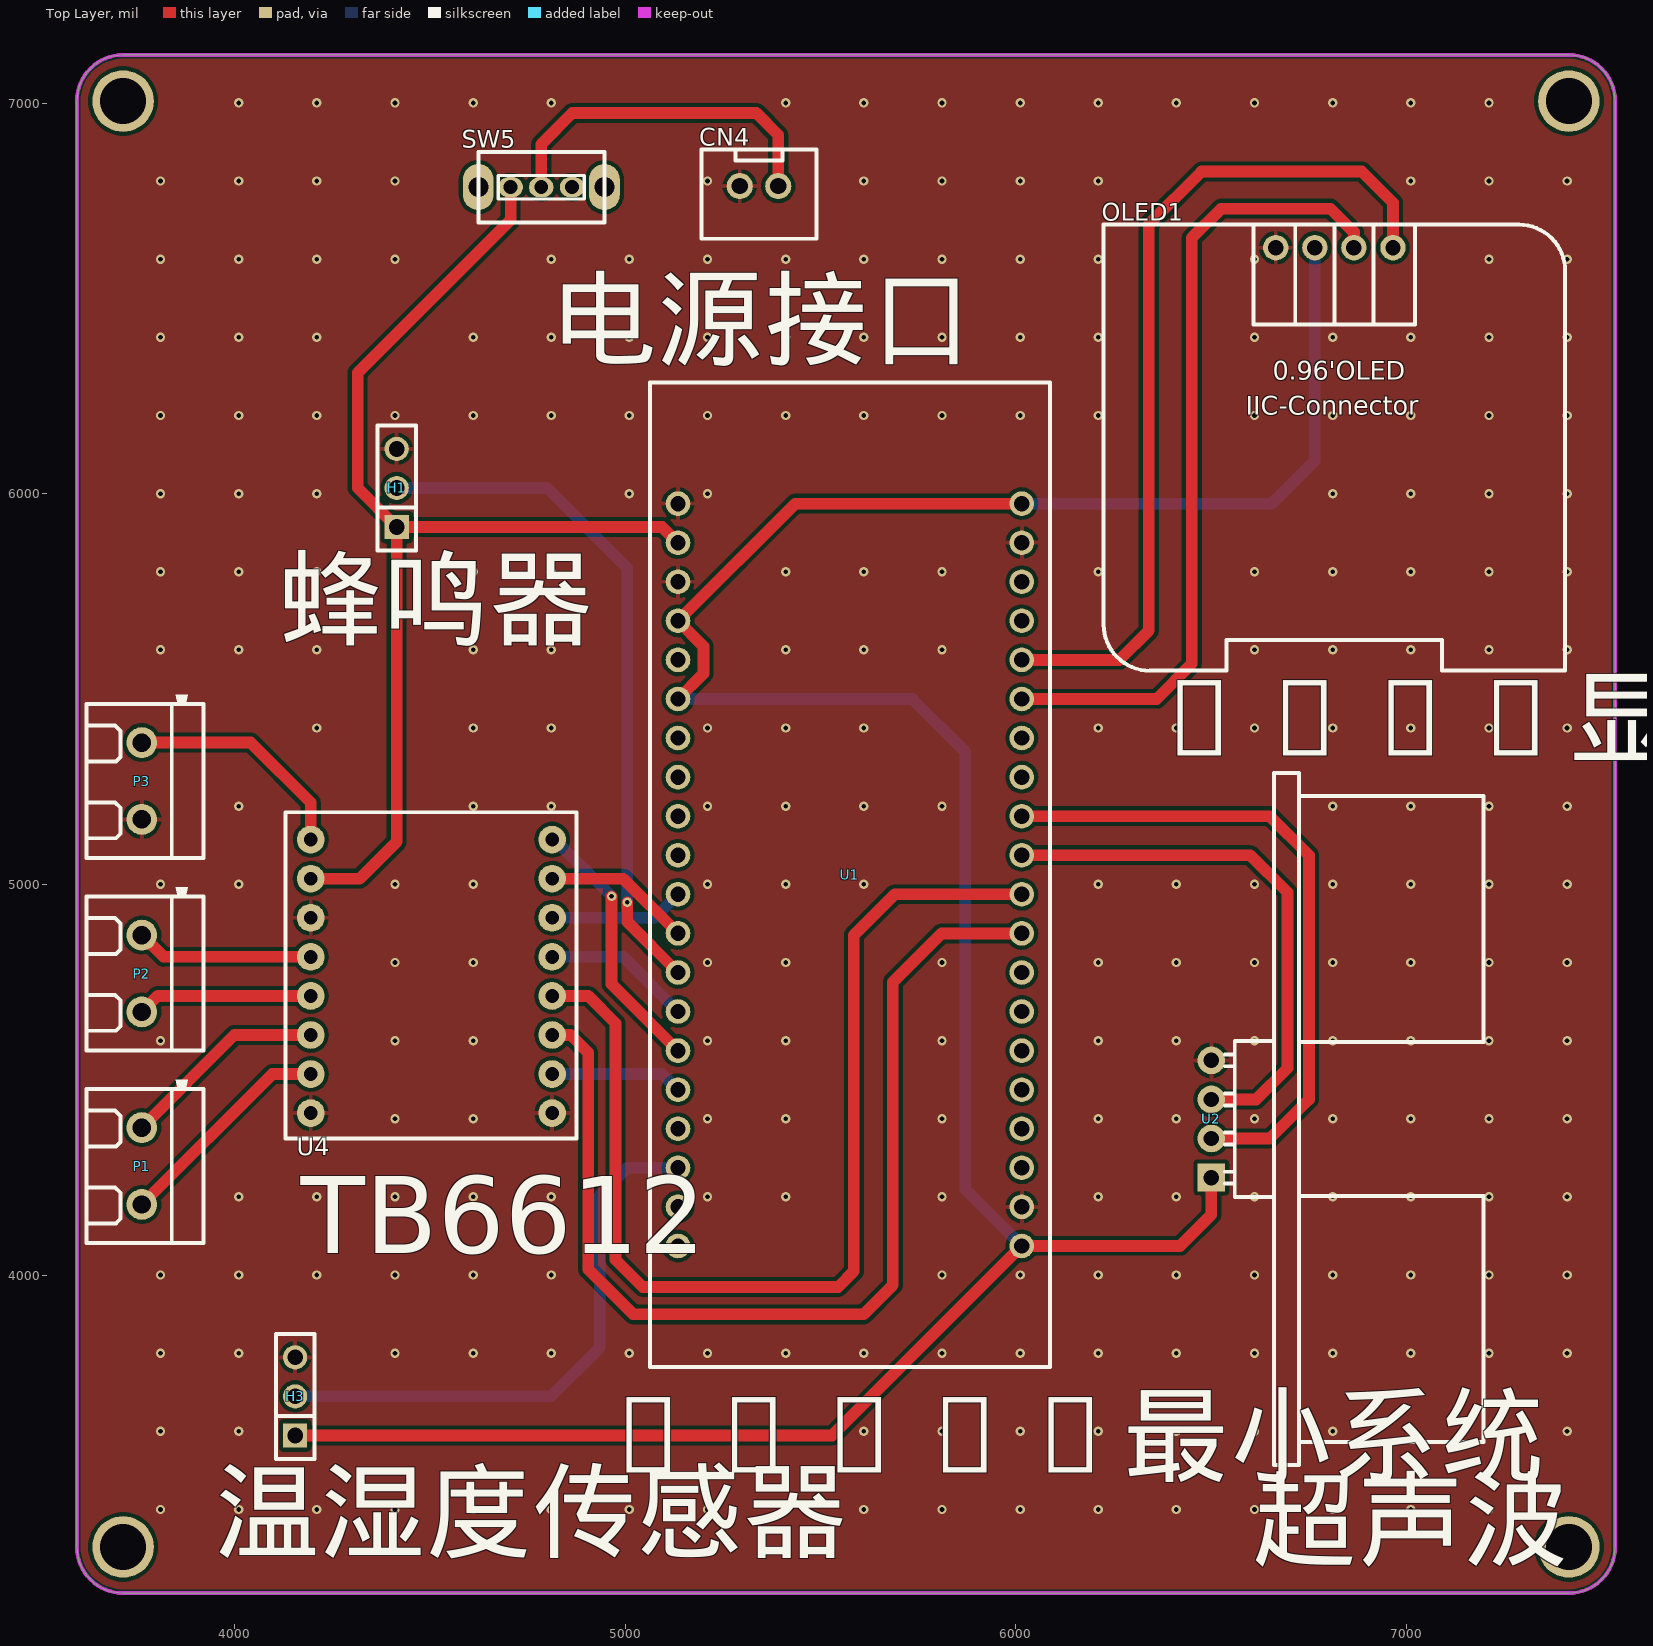
[diagram p0: Top Layer view]
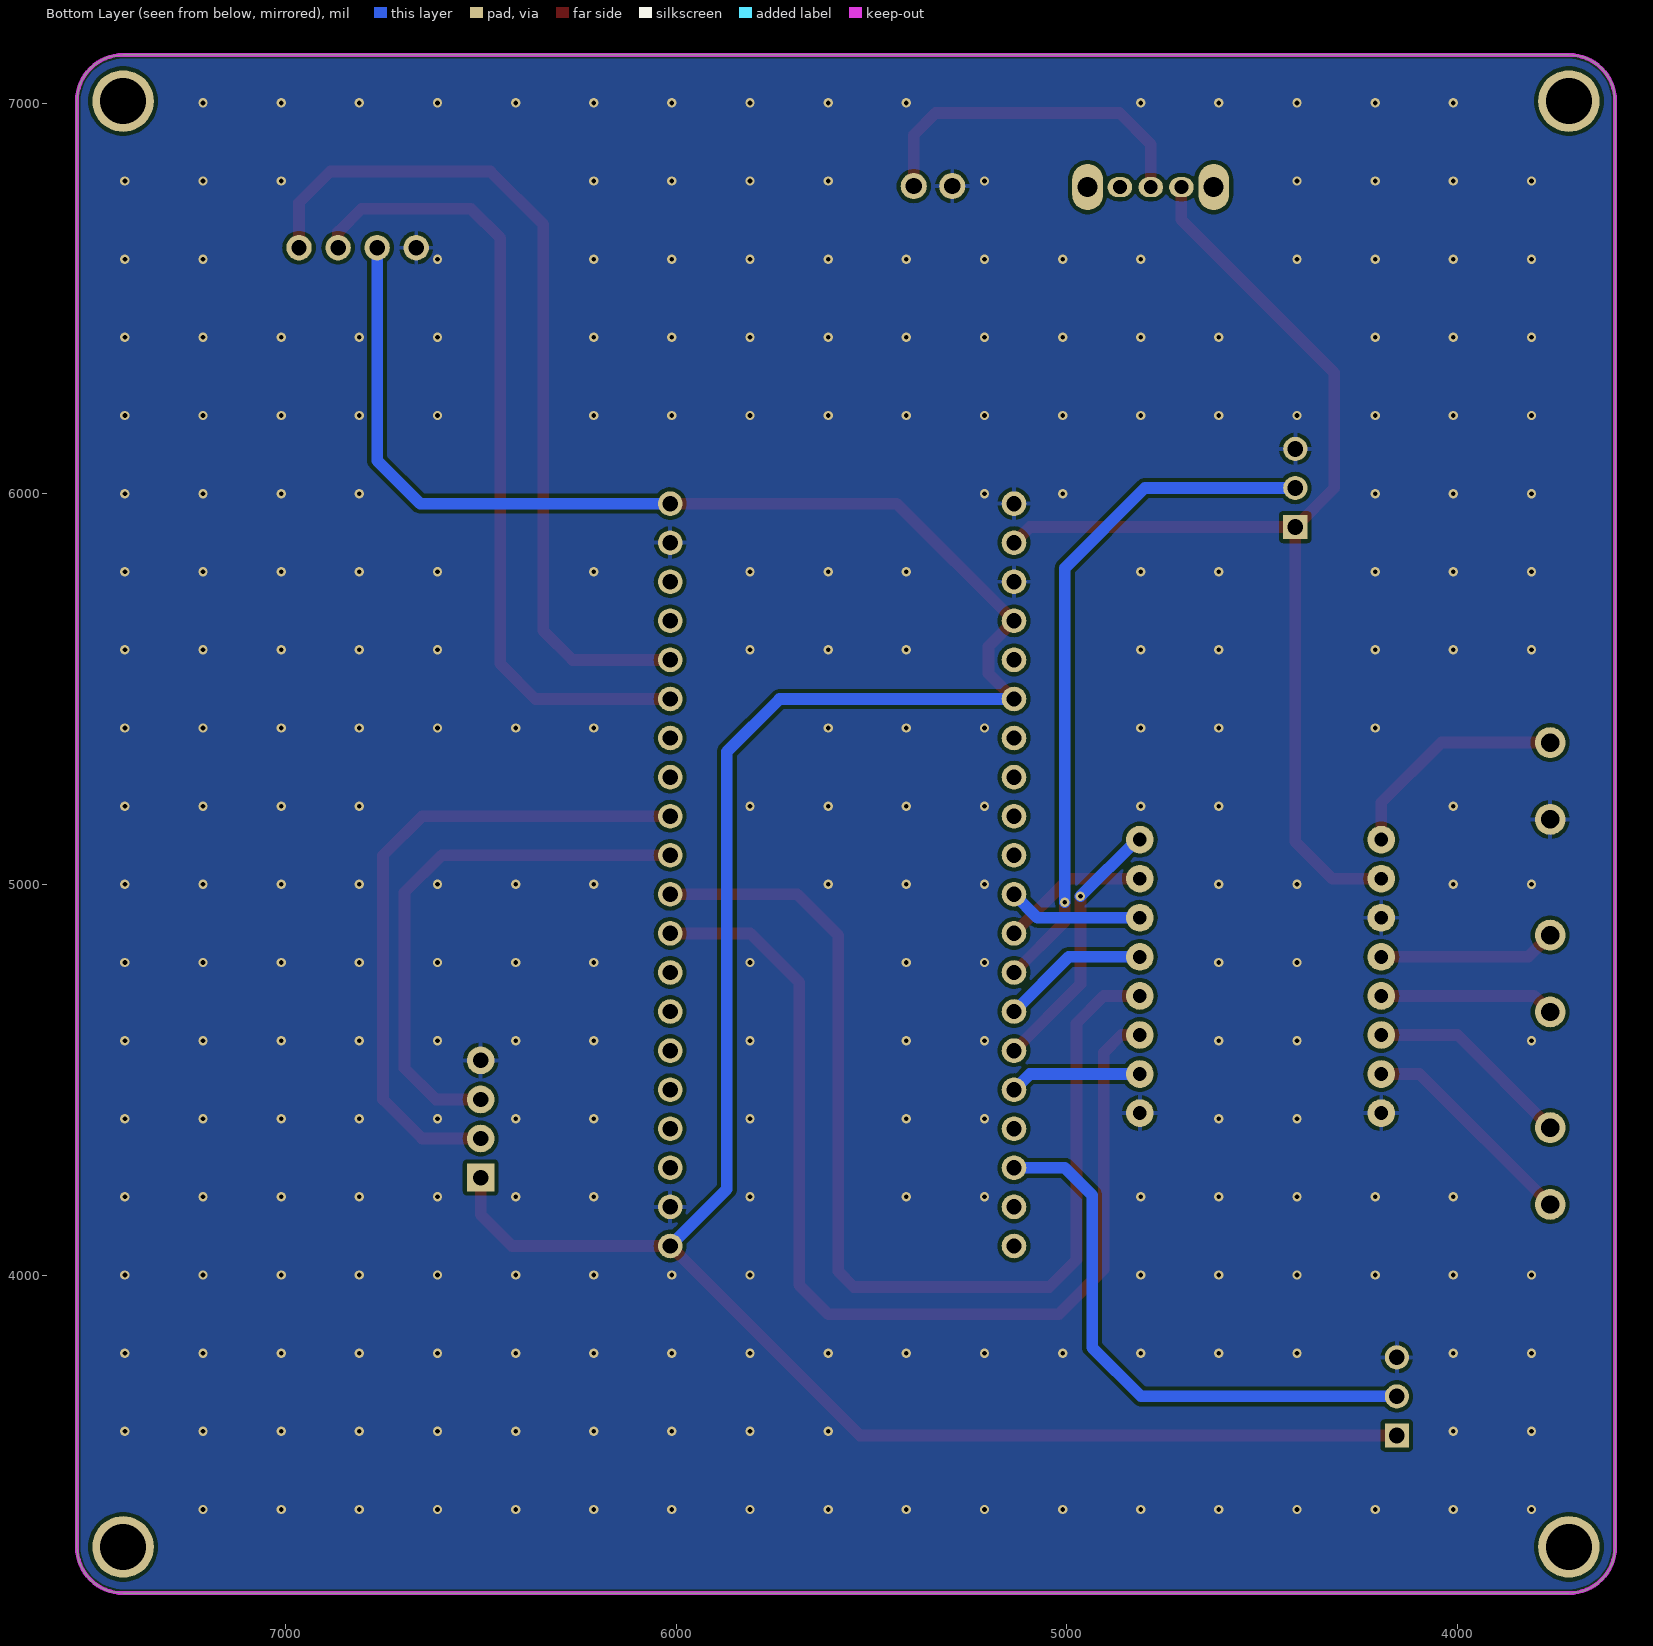
[diagram p1: Bottom Layer view, seen from below]
# Altium PCB MISC52080.pcbdoc
Units mil, origin at the board's own origin, x right, y up, seen from the top; angles counter-clockwise.
Board outline 3937.01 x 3937.01 mil, 2 copper layers (Top Layer, Bottom Layer), stack 62.206 mil thick; 11 components, 40 nets, 87 pads, 268 vias.

## Layer stack, top to bottom
Top Solder Mask Layer: solder mask 0.394, Dk 3.3
Top Layer: signal copper 1.379
Dielectric1: surface 59.449, FR4, Dk 4.5
Bottom Layer: signal copper 1.378
Bottom Solder Mask Layer: solder mask 0.394, Dk 3.3

## Board outline
3714.61,7123.5 ccw(c3714.61,7005.39) 3596.5,7005.39 3596.5,3304.61 ccw(c3714.61,3304.61) 3714.61,3186.5 7415.39,3186.5 ccw(c7415.39,3304.61) 7533.5,3304.61 7533.5,7005.39 ccw(c7415.39,7005.39) 7415.39,7123.5 3714.61,7123.5

## Design rules (kind name [scope] priority, off if disabled: settings)
BoardOutlineClearance copperThickness2oz_1 [All] p2 off: genericclearance=7.99 ignorepadtopadclearanceinfootprint=FALSE except(0: Arc-SplitContinuation Track-SplitContinuation SMDPad-SplitContinuation THPad-SplitContinuation Via-SplitContinuation Fill-SplitContinuation Region-SplitContinuation Poly-SplitContinuation Text-SplitContinuation Hole-SplitContinuation; 5.98: Arc-CutoutEdge Track-CutoutEdge SMDPad-CutoutEdge THPad-CutoutEdge Via-CutoutEdge Text-CutoutEdge; 6.9: Hole-OutlineEdge Hole-CutoutEdge; 10: Poly-OutlineEdge Poly-CutoutEdge; 11.81: Arc-OutlineEdge Track-OutlineEdge SMDPad-OutlineEdge THPad-OutlineEdge Via-OutlineEdge Fill-OutlineEdge Region-OutlineEdge Text-OutlineEdge Fill-CutoutEdge Region-CutoutEdge)
BoardOutlineClearance Plane_innerPlane_1 [All] p4 off: genericclearance=4.02 ignorepadtopadclearanceinfootprint=FALSE except(0: Arc-SplitContinuation Track-SplitContinuation SMDPad-SplitContinuation THPad-SplitContinuation Via-SplitContinuation Fill-SplitContinuation Region-SplitContinuation Poly-SplitContinuation Text-SplitContinuation Hole-SplitContinuation; 5.98: Arc-CutoutEdge Track-CutoutEdge SMDPad-CutoutEdge THPad-CutoutEdge Via-CutoutEdge Text-CutoutEdge; 6.9: Hole-OutlineEdge Hole-CutoutEdge; 10: Poly-OutlineEdge Poly-CutoutEdge; 11.81: Arc-OutlineEdge Track-OutlineEdge SMDPad-OutlineEdge THPad-OutlineEdge Via-OutlineEdge Fill-OutlineEdge Region-OutlineEdge Text-OutlineEdge Fill-CutoutEdge Region-CutoutEdge)
BoardOutlineClearance Copper_copperRegion_1 [All] p6 off: genericclearance=4.02 ignorepadtopadclearanceinfootprint=FALSE except(0: Arc-SplitContinuation Track-SplitContinuation SMDPad-SplitContinuation THPad-SplitContinuation Via-SplitContinuation Fill-SplitContinuation Region-SplitContinuation Poly-SplitContinuation Text-SplitContinuation Hole-SplitContinuation; 5.98: Arc-CutoutEdge Track-CutoutEdge SMDPad-CutoutEdge THPad-CutoutEdge Via-CutoutEdge Text-CutoutEdge; 6.9: Hole-OutlineEdge Hole-CutoutEdge; 10: Poly-OutlineEdge Poly-CutoutEdge; 11.81: Arc-OutlineEdge Track-OutlineEdge SMDPad-OutlineEdge THPad-OutlineEdge Via-OutlineEdge Fill-OutlineEdge Region-OutlineEdge Text-OutlineEdge Fill-CutoutEdge Region-CutoutEdge)
BoardOutlineClearance Copper_copperRegion_copperThickness1oz_1 [All] p8 off: genericclearance=4.02 ignorepadtopadclearanceinfootprint=FALSE except(0: Arc-SplitContinuation Track-SplitContinuation SMDPad-SplitContinuation THPad-SplitContinuation Via-SplitContinuation Fill-SplitContinuation Region-SplitContinuation Poly-SplitContinuation Text-SplitContinuation Hole-SplitContinuation; 5.98: Arc-CutoutEdge Track-CutoutEdge SMDPad-CutoutEdge THPad-CutoutEdge Via-CutoutEdge Text-CutoutEdge; 6.9: Hole-OutlineEdge Hole-CutoutEdge; 10: Poly-OutlineEdge Poly-CutoutEdge; 11.81: Arc-OutlineEdge Track-OutlineEdge SMDPad-OutlineEdge THPad-OutlineEdge Via-OutlineEdge Fill-OutlineEdge Region-OutlineEdge Text-OutlineEdge Fill-CutoutEdge Region-CutoutEdge)
BoardOutlineClearance Copper_copperRegion_Copper_copperRegion_1 [All] p10 off: genericclearance=4.02 ignorepadtopadclearanceinfootprint=FALSE except(0: Arc-SplitContinuation Track-SplitContinuation SMDPad-SplitContinuation THPad-SplitContinuation Via-SplitContinuation Fill-SplitContinuation Region-SplitContinuation Poly-SplitContinuation Text-SplitContinuation Hole-SplitContinuation; 5.98: Arc-CutoutEdge Track-CutoutEdge SMDPad-CutoutEdge THPad-CutoutEdge Via-CutoutEdge Text-CutoutEdge; 6.9: Hole-OutlineEdge Hole-CutoutEdge; 10: Poly-OutlineEdge Poly-CutoutEdge; 11.81: Arc-OutlineEdge Track-OutlineEdge SMDPad-OutlineEdge THPad-OutlineEdge Via-OutlineEdge Fill-OutlineEdge Region-OutlineEdge Text-OutlineEdge Fill-CutoutEdge Region-CutoutEdge)
BoardOutlineClearance copperThickness1oz_1 [All] p12: genericclearance=4.02 ignorepadtopadclearanceinfootprint=FALSE except(0: Arc-SplitContinuation Track-SplitContinuation SMDPad-SplitContinuation THPad-SplitContinuation Via-SplitContinuation Fill-SplitContinuation Region-SplitContinuation Poly-SplitContinuation Text-SplitContinuation Hole-SplitContinuation; 5.98: Arc-CutoutEdge Track-CutoutEdge SMDPad-CutoutEdge THPad-CutoutEdge Via-CutoutEdge Text-CutoutEdge; 6.9: Hole-OutlineEdge Hole-CutoutEdge; 10: Poly-OutlineEdge Poly-CutoutEdge; 11.81: Arc-OutlineEdge Track-OutlineEdge SMDPad-OutlineEdge THPad-OutlineEdge Via-OutlineEdge Fill-OutlineEdge Region-OutlineEdge Text-OutlineEdge Fill-CutoutEdge Region-CutoutEdge)
Clearance copperThickness2oz [All] p1 off: gap=7.99 ignorepadtopadclearanceinfootprint=FALSE except(5.98: SMDPad-Track SMDPad-SMDPad THPad-Track SMDPad-THPad THPad-THPad Track-Via SMDPad-Via THPad-Via Via-Via Fill-SMDPad Region-SMDPad Fill-THPad Region-THPad Fill-Via Region-Via Fill-Fill Fill-Region Region-Region Arc-Track Arc-SMDPad Arc-THPad Arc-Via Fill-Arc Region-Arc Arc-Arc Text-Track SMDPad-Text Text-THPad Text-Via Fill-Text Region-Text Arc-Text Text-Text; 6.9: Hole-Track Hole-SMDPad Hole-THPad Hole-Via Fill-Hole Region-Hole Hole-Arc Hole-Text; 10: Poly-Track Poly-SMDPad Poly-THPad Poly-Via Poly-Fill Poly-Region Poly-Poly Poly-Arc Poly-Text Poly-Hole; 11.81: Fill-Track Region-Track)
Clearance Plane_innerPlane [All] p3 off: gap=4.02 ignorepadtopadclearanceinfootprint=FALSE except(5.98: SMDPad-Track SMDPad-SMDPad THPad-Track SMDPad-THPad THPad-THPad Track-Via SMDPad-Via THPad-Via Via-Via Fill-SMDPad Region-SMDPad Fill-THPad Region-THPad Fill-Via Region-Via Fill-Fill Fill-Region Region-Region Arc-Track Arc-SMDPad Arc-THPad Arc-Via Fill-Arc Region-Arc Arc-Arc Text-Track SMDPad-Text Text-THPad Text-Via Fill-Text Region-Text Arc-Text Text-Text; 6.9: Hole-Track Hole-SMDPad Hole-THPad Hole-Via Fill-Hole Region-Hole Hole-Arc Hole-Text; 10: Poly-Track Poly-SMDPad Poly-THPad Poly-Via Poly-Fill Poly-Region Poly-Poly Poly-Arc Poly-Text Poly-Hole; 11.81: Fill-Track Region-Track)
Clearance Copper_copperRegion [All] p5 off: gap=4.02 ignorepadtopadclearanceinfootprint=FALSE except(5.98: SMDPad-Track SMDPad-SMDPad THPad-Track SMDPad-THPad THPad-THPad Track-Via SMDPad-Via THPad-Via Via-Via Fill-SMDPad Region-SMDPad Fill-THPad Region-THPad Fill-Via Region-Via Fill-Fill Fill-Region Region-Region Arc-Track Arc-SMDPad Arc-THPad Arc-Via Fill-Arc Region-Arc Arc-Arc Text-Track SMDPad-Text Text-THPad Text-Via Fill-Text Region-Text Arc-Text Text-Text; 6.9: Hole-Track Hole-SMDPad Hole-THPad Hole-Via Fill-Hole Region-Hole Hole-Arc Hole-Text; 10: Poly-Track Poly-SMDPad Poly-THPad Poly-Via Poly-Fill Poly-Region Poly-Poly Poly-Arc Poly-Text Poly-Hole; 11.81: Fill-Track Region-Track)
Clearance Copper_copperRegion_copperThickness1oz [All] p7 off: gap=4.02 ignorepadtopadclearanceinfootprint=FALSE except(5.98: SMDPad-Track SMDPad-SMDPad THPad-Track SMDPad-THPad THPad-THPad Track-Via SMDPad-Via THPad-Via Via-Via Fill-SMDPad Region-SMDPad Fill-THPad Region-THPad Fill-Via Region-Via Fill-Fill Fill-Region Region-Region Arc-Track Arc-SMDPad Arc-THPad Arc-Via Fill-Arc Region-Arc Arc-Arc Text-Track SMDPad-Text Text-THPad Text-Via Fill-Text Region-Text Arc-Text Text-Text; 6.9: Hole-Track Hole-SMDPad Hole-THPad Hole-Via Fill-Hole Region-Hole Hole-Arc Hole-Text; 10: Poly-Track Poly-SMDPad Poly-THPad Poly-Via Poly-Fill Poly-Region Poly-Poly Poly-Arc Poly-Text Poly-Hole; 11.81: Fill-Track Region-Track)
Clearance Copper_copperRegion_Copper_copperRegion [All] p9 off: gap=4.02 ignorepadtopadclearanceinfootprint=FALSE except(5.98: SMDPad-Track SMDPad-SMDPad THPad-Track SMDPad-THPad THPad-THPad Track-Via SMDPad-Via THPad-Via Via-Via Fill-SMDPad Region-SMDPad Fill-THPad Region-THPad Fill-Via Region-Via Fill-Fill Fill-Region Region-Region Arc-Track Arc-SMDPad Arc-THPad Arc-Via Fill-Arc Region-Arc Arc-Arc Text-Track SMDPad-Text Text-THPad Text-Via Fill-Text Region-Text Arc-Text Text-Text; 6.9: Hole-Track Hole-SMDPad Hole-THPad Hole-Via Fill-Hole Region-Hole Hole-Arc Hole-Text; 10: Poly-Track Poly-SMDPad Poly-THPad Poly-Via Poly-Fill Poly-Region Poly-Poly Poly-Arc Poly-Text Poly-Hole; 11.81: Fill-Track Region-Track)
Clearance copperThickness1oz [All] p11: gap=4.02 ignorepadtopadclearanceinfootprint=FALSE except(5.98: SMDPad-Track SMDPad-SMDPad THPad-Track SMDPad-THPad THPad-THPad Track-Via SMDPad-Via THPad-Via Via-Via Fill-SMDPad Region-SMDPad Fill-THPad Region-THPad Fill-Via Region-Via Fill-Fill Fill-Region Region-Region Arc-Track Arc-SMDPad Arc-THPad Arc-Via Fill-Arc Region-Arc Arc-Arc Text-Track SMDPad-Text Text-THPad Text-Via Fill-Text Region-Text Arc-Text Text-Text; 6.9: Hole-Track Hole-SMDPad Hole-THPad Hole-Via Fill-Hole Region-Hole Hole-Arc Hole-Text; 10: Poly-Track Poly-SMDPad Poly-THPad Poly-Via Poly-Fill Poly-Region Poly-Poly Poly-Arc Poly-Text Poly-Hole; 11.81: Fill-Track Region-Track)
DiffPairsRouting differentialPair [All] p1: maxlimit=6 minlimit=6 mostfreqgap=6 toplayer_minwidth=5 toplayer_prefwidth=10 toplayer_maxwidth=100 toplayer_mingap=6 toplayer_prefgap=6 toplayer_maxgap=6 bottomlayer_minwidth=5 bottomlayer_prefwidth=10 bottomlayer_maxwidth=100 bottomlayer_mingap=6 bottomlayer_prefgap=6 bottomlayer_maxgap=6 maxuncoupledlength=10
HoleToHoleClearance otherClearance [All] p1: gap=11.81 allowstackedmicrovias=TRUE
Length netLength [All] p1: minlimit=0 maxlimit=0
PasteMaskExpansion pasteMaskExpansion [All] p1: expansion=0
PlaneConnect innerPlane [All] p1: planeconnectstyle=Relief reliefexpansion=20 reliefentries=4 reliefconductorwidth=10 reliefairgap=10
PolygonConnect copperRegion_copperThickness1oz [All] p1 off: connectstyle=Relief reliefconductorwidth=10 reliefentries=4 polygonreliefangle="90 Angle" airgapwidth=10 via.connectstyle=Relief via.reliefconductorwidth=10 via.reliefentries=4 via.polygonreliefangle="90 Angle" via.airgapwidth=10
PolygonConnect copperRegion_Copper_copperRegion [All] p2 off: connectstyle=Relief reliefconductorwidth=10 reliefentries=4 polygonreliefangle="90 Angle" airgapwidth=10 via.connectstyle=Relief via.reliefconductorwidth=10 via.reliefentries=4 via.polygonreliefangle="90 Angle" via.airgapwidth=10
PolygonConnect copperRegion [All] p3: connectstyle=Relief reliefconductorwidth=10 reliefentries=4 polygonreliefangle="90 Angle" airgapwidth=10 via.connectstyle=Relief via.reliefconductorwidth=10 via.reliefentries=4 via.polygonreliefangle="90 Angle" via.airgapwidth=10
RoutingVias viaSize [All] p1: holewidth=12.01 width=24.02 viastyle="Through Hole" minholewidth=11.81 minwidth=19.68 maxholewidth=248.03 maxwidth=393.7
SolderMaskExpansion solderMaskExpansion [IsVia] p1: expansion=-1000 istentingtop=TRUE
SolderMaskExpansion solderMaskExpansion [All] p2: expansion=2 istentingtop=FALSE
Width copperThickness2oz_2 [All] p1 off: maxlimit=100 minlimit=8 preferedwidth=10
Width copperThickness1oz_2 [All] p2: maxlimit=100 minlimit=5 preferedwidth=10

## Components (designator, comment, footprint, x,y, rotation, side; value= is the part's Value field where it differs from the comment)
CN4 "XH2.54*2P_直插" CONN-TH_2P-P2.50-XH2.54-2P 5342.32,6787.68 r0 top
H1 "" HDR-TH_3P-P2.54-V-F 4415,6015 r90 top
H3 "" HDR-TH_3P-P2.54-V-F 4155,3690 r90 top
OLED1 "" 0.96OLED_4P 6815,6630 r0 top
P1 "KF301-2P接线端子" CONN-TH_XY301V-A-5.0-2P 3762.74,4279.59 r90 top
P2 "KF301-2P接线端子" CONN-TH_XY301V-A-5.0-2P 3762.74,4772.29 r90 top
P3 "KF301-2P接线端子" CONN-TH_XY301V-A-5.0-2P 3762.74,5265 r90 top
SW5 "" 拨动开关 4780,6785 r0 top
U1 "STM32F103C8T6-Card" CONN-TH_L53.3-W22.9_STM32F103C8T6-CARD 5575,5025 r90 top
U2 "HC-SR04" TH_HC-SR04V 6500,4400 r90 top
U4 "" tb6612 4195,5115 r0 top

## Footprints (in the part's own frame and the unit in brackets; to place one, negate y for a bottom-side part, rotate by r counter-clockwise, add the part's x,y. Pads: shape width x height; smd on the part's side, far side on the other; paste and mask are expansions set on the pad)
0.96OLED_4P [mm]
  round 1.65 hole 1 copper offset 0,0: 1(-3.81,-0.001) 2(-1.27,0.002) 3(1.27,0.002) 4(3.81,0.002)
  silkscreen extent -15,-27.5 15,1.5
CONN-TH_2P-P2.50-XH2.54-2P [mm]
  round 1.7 hole 1.05 paste+0 mask+0.05: 1(1.25,0) 2(-1.25,0)
  silkscreen extent -3.75,-3.42 3.75,2.37
CONN-TH_L53.3-W22.9_STM32F103C8T6-CARD [mm]
  round 1.6 hole 1: 1(-24.13,-11.176) 2(-21.59,-11.176) 3(-19.05,-11.176) 4(-16.51,-11.176) 5(-13.97,-11.176) 6(-11.43,-11.176) 7(-8.89,-11.176) 8(-6.35,-11.176) 9(-3.81,-11.176) 10(-1.27,-11.176) 11(1.27,-11.176) 12(3.81,-11.176) 13(6.35,-11.176) 14(8.89,-11.176) 15(11.43,-11.176) 16(13.97,-11.176) 17(16.51,-11.176) 18(19.05,-11.176) 19(21.59,-11.176) 20(24.13,-11.176) 21(24.13,11.176) 22(21.59,11.176) 23(19.05,11.176) 24(16.51,11.176) 25(13.97,11.176) 26(11.43,11.176) 27(8.89,11.176) 28(6.35,11.176) 29(3.81,11.176) 30(1.27,11.176) 31(-1.27,11.176) 32(-3.81,11.176) 33(-6.35,11.176) 34(-8.89,11.176) 35(-11.43,11.176) 36(-13.97,11.176) 37(-16.51,11.176) 38(-19.05,11.176) 39(-21.59,11.176) 40(-24.13,11.176)
  silkscreen extent -32,-13 32,13
CONN-TH_XY301V-A-5.0-2P [mm]
  round 2 hole 1.2: 1(-2.5,0) 2(2.5,0)
  silkscreen extent -5,-4 5.6,3.6
HDR-TH_3P-P2.54-V-F [mil]
  rect 62x62 hole 40.16: 1(-100,0)
  round 62 hole 40.16: 2(0,0) 3(100,0)
  silkscreen extent -160,-49 160,49
tb6612 [mm]
  round 1.8 hole 0.9: 1(0,0) 2(0,-2.54) 3(0,-5.08) 4(0,-7.62) 5(0,-10.16) 6(0,-12.7) 7(0,-15.24) 8(0,-17.78) 9(15.697,-17.78) 10(15.697,-15.24) 11(15.697,-12.7) 12(15.697,-10.16) 13(15.697,-7.62) 14(15.697,-5.08) 15(15.697,-2.54) 16(15.697,0)
  silkscreen extent -1.65,-19.43 17.27,1.78
TH_HC-SR04V [mm]
  rect 1.8x1.8 hole 1.001: 1(-3.81,0)
  round 1.8 hole 1.001: 2(-1.27,0) 3(1.27,0) 4(3.81,0)
  silkscreen extent -22.5,-17.7 22.5,-0.89
拨动开关 [mil]
  oval 63x51.2 hole 35.4 paste+0 mask+2: 1(-73.4,0) 2(5,0) 3(84,0)
  oval 78.7x118.1 hole 51.2 paste+0 mask+2: 4(166.7,0) 5(-156.1,0)
  silkscreen extent -156,-90 167,90

## Free pads (board coordinates)
  round 157.48 hole 118.11: 1(3714.61,7005.39) 1(3714.61,3304.61) 1(7415.39,7005.39) 1(7415.39,3304.61)

## Via types
v1: diameter 24.02, hole 12, Top Layer to Bottom Layer, 268 vias

## Nets (pads, with @x,y where several pads share a name; then routed paths per layer and width w, separated by ;. In a path a pad name is that pad's centre, name@x,y a point inside that pad or via, vN(x,y) a via of type N, cw(c..) or ccw(c..) an arc to the next point about the centre after c; other vN are vias at no path point)
$1N17219: P2.2 U4.4 | length 455.3
  Top Layer w30: P2.2 3818.46,4815 U4.4
$1N17220: P2.1 U4.5 | length 449.3
  Top Layer w30: P2.1 3803.87,4715 U4.5
$1N17221: P1.2 U4.6 | length 530.4
  Top Layer w30: P1.2 3999.73,4615 U4.6
$1N17222: P1.1 U4.7 | length 570.5
  Top Layer w30: P1.1 4096.58,4515 U4.7
$1N17227: CN4.1 SW5.2 | length 903.9
  Top Layer w30: SW5.2 4785,6895 4865,6975 5335,6975 5391.54,6918.46 CN4.1
+5V: H1.1 SW5.1 U1.22 U4.2 | length 2874.5
  Top Layer w30: U4.2 4320,5015 4415,5110 H1.1 ; SW5.1 4706.6,6701.6 4315,6310 4315,6015 H1.1 ; U1.22 5095,5915 H1.1
GND: CN4.2 H1.3 H3.3 OLED1.1 P3.1 U1.2 U1.19 U1.21 U1.23 U2.4 U4.3 U4.8 U4.9
  other v1: 3810.6,3400.6 4010.6,3400.6 4210.6,3400.6 4410.6,3400.6 4610.6,3400.6 4810.6,3400.6 5010.6,3400.6 5210.6,3400.6 5410.6,3400.6 5610.6,3400.6 5810.6,3400.6 6010.6,3400.6 6210.6,3400.6 6410.6,3400.6 6610.6,3400.6 6810.6,3400.6 7010.6,3400.6 7210.6,3400.6 3810.6,3600.6 4010.6,3600.6 5610.6,3600.6 5810.6,3600.6 6010.6,3600.6 6210.6,3600.6 6410.6,3600.6 6610.6,3600.6 6810.6,3600.6 7010.6,3600.6 7210.6,3600.6 7410.6,3600.6 3810.6,3800.6 4010.6,3800.6 4410.6,3800.6 4610.6,3800.6 4810.6,3800.6 5010.6,3800.6 5210.6,3800.6 5410.6,3800.6 5610.6,3800.6 5810.6,3800.6 6010.6,3800.6 6210.6,3800.6 6410.6,3800.6 6610.6,3800.6 6810.6,3800.6 7010.6,3800.6 7210.6,3800.6 7410.6,3800.6 3810.6,4000.6 4010.6,4000.6 4210.6,4000.6 4410.6,4000.6 4610.6,4000.6 4810.6,4000.6 5810.6,4000.6 6010.6,4000.6 6210.6,4000.6 6410.6,4000.6 6610.6,4000.6 6810.6,4000.6 7010.6,4000.6 7210.6,4000.6 7410.6,4000.6 4010.6,4200.6 4210.6,4200.6 4410.6,4200.6 4610.6,4200.6 4810.6,4200.6 5210.6,4200.6 5410.6,4200.6 5810.6,4200.6 6210.6,4200.6 6410.6,4200.6 6610.6,4200.6 6810.6,4200.6 7010.6,4200.6 7210.6,4200.6 7410.6,4200.6 4410.6,4400.6 4610.6,4400.6 5210.6,4400.6 5410.6,4400.6 5810.6,4400.6 6210.6,4400.6 6410.6,4400.6 6610.6,4400.6 6810.6,4400.6 7010.6,4400.6 7210.6,4400.6 7410.6,4400.6 3810.6,4600.6 4410.6,4600.6 4610.6,4600.6 5210.6,4600.6 5410.6,4600.6 5810.6,4600.6 6210.6,4600.6 6410.6,4600.6 6610.6,4600.6 6810.6,4600.6 7010.6,4600.6 7210.6,4600.6 7410.6,4600.6 4410.6,4800.6 4610.6,4800.6 5210.6,4800.6 5410.6,4800.6 5810.6,4800.6 6210.6,4800.6 6410.6,4800.6 6610.6,4800.6 6810.6,4800.6 7010.6,4800.6 7210.6,4800.6 7410.6,4800.6 3810.6,5000.6 4010.6,5000.6 4410.6,5000.6 4610.6,5000.6 5210.6,5000.6 5410.6,5000.6 5610.6,5000.6 6210.6,5000.6 6410.6,5000.6 6610.6,5000.6 6810.6,5000.6 7010.6,5000.6 7210.6,5000.6 7410.6,5000.6 4010.6,5200.6 4610.6,5200.6 4810.6,5200.6 5210.6,5200.6 5410.6,5200.6 5610.6,5200.6 5810.6,5200.6 6810.6,5200.6 7010.6,5200.6 7210.6,5200.6 7410.6,5200.6 4210.6,5400.6 4610.6,5400.6 4810.6,5400.6 5210.6,5400.6 5410.6,5400.6 5610.6,5400.6 6210.6,5400.6 6410.6,5400.6 6610.6,5400.6 6810.6,5400.6 7010.6,5400.6 7210.6,5400.6 7410.6,5400.6 3810.6,5600.6 4010.6,5600.6 4210.6,5600.6 4610.6,5600.6 4810.6,5600.6 5410.6,5600.6 5610.6,5600.6 5810.6,5600.6 6610.6,5600.6 6810.6,5600.6 7010.6,5600.6 7210.6,5600.6 7410.6,5600.6 3810.6,5800.6 4010.6,5800.6 4210.6,5800.6 4610.6,5800.6 4810.6,5800.6 5410.6,5800.6 5610.6,5800.6 5810.6,5800.6 6210.6,5800.6 6610.6,5800.6 6810.6,5800.6 7010.6,5800.6 7210.6,5800.6 7410.6,5800.6 3810.6,6000.6 4010.6,6000.6 4210.6,6000.6 5010.6,6000.6 5210.6,6000.6 6810.6,6000.6 7010.6,6000.6 7210.6,6000.6 7410.6,6000.6 3810.6,6200.6 4010.6,6200.6 4210.6,6200.6 4410.6,6200.6 4610.6,6200.6 4810.6,6200.6 5010.6,6200.6 5210.6,6200.6 5410.6,6200.6 5610.6,6200.6 5810.6,6200.6 6010.6,6200.6 6210.6,6200.6 6610.6,6200.6 6810.6,6200.6 7010.6,6200.6 7210.6,6200.6 7410.6,6200.6 3810.6,6400.6 4010.6,6400.6 4210.6,6400.6 4610.6,6400.6 4810.6,6400.6 5010.6,6400.6 5210.6,6400.6 5410.6,6400.6 5610.6,6400.6 5810.6,6400.6 6010.6,6400.6 6210.6,6400.6 6610.6,6400.6 6810.6,6400.6 7010.6,6400.6 7210.6,6400.6 7410.6,6400.6 3810.6,6600.6 4010.6,6600.6 4210.6,6600.6 4410.6,6600.6 4810.6,6600.6 5010.6,6600.6 5210.6,6600.6 5410.6,6600.6 5610.6,6600.6 5810.6,6600.6 6010.6,6600.6 6210.6,6600.6 6610.6,6600.6 7210.6,6600.6 7410.6,6600.6 3810.6,6800.6 4010.6,6800.6 4210.6,6800.6 4410.6,6800.6 5210.6,6800.6 5610.6,6800.6 5810.6,6800.6 6010.6,6800.6 6210.6,6800.6 7010.6,6800.6 7210.6,6800.6 7410.6,6800.6 4010.6,7000.6 4210.6,7000.6 4410.6,7000.6 4610.6,7000.6 4810.6,7000.6 5410.6,7000.6 5610.6,7000.6 5810.6,7000.6 6010.6,7000.6 6210.6,7000.6 6410.6,7000.6 6610.6,7000.6 6810.6,7000.6 7010.6,7000.6 7210.6,7000.6
PA0: U1.27
PA1: U1.28
PA2: U1.29
PA3: U1.30
PA4: U1.31 U4.14 | length 346.9
  Bottom Layer w30: U4.14 5075,4915 U1.31
PA5: U1.32 U4.15 | length 380
  Top Layer w30: U4.15 4995,5015 U1.32
PA6: H1.2 U1.33 | length 1763.8
  Top Layer w30: v1(5005,4955) 5005,4905 U1.33
  Bottom Layer w30: H1.2 4800,6015 5005,5810 v1(5005,4955)
PA7: U1.34 U4.13 | length 380
  Bottom Layer w30: U4.13 4995,4815 U1.34
PA8: U1.7
PA9: U1.5
PA10: U1.6
PA11: U1.3
PA12: U1.4
PA15: U1.11 U2.3 | length 1397.5
  Top Layer w30: U1.11 6600,5075 6695,4980 6695,4530 6615,4450 U2.3
PB0: U1.35 U4.16 | length 677.5
  Top Layer w30: v1(4965,4970) 4965,4745 U1.35
  Bottom Layer w30: U4.16 4820,5115 v1(4965,4970)
PB1: U1.36 U4.10 | length 338.6
  Bottom Layer w30: U4.10 5095,4515 U1.36
PB3: U1.12 U2.2 | length 1692.8
  Top Layer w30: U1.12 6650,5175 6750,5075 6750,4450 6650,4350 U2.2
PB4: U1.13
PB5: U1.14
PB6: OLED1.3 U1.15 | length 2073.1
  Top Layer w30: U1.15 6360,5475 6450,5565 6450,6655 6525,6730 6805,6730 6865,6670 OLED1.3@6865,6630.05
PB7: OLED1.4 U1.16 | length 2225.1
  Top Layer w30: U1.16 6265,5575 6340,5650 6340,6690 6475,6825 6885,6825 6965,6745 OLED1.4@6965,6630.05
PB8: U1.17
PB9: U1.18
PB10: U1.37
PB11: H3.2 U1.38 | length 1450.8
  Bottom Layer w30: H3.2 4810,3690 4935,3815 4935,4205 5005,4275 U1.38
PB12: U1.39
PB13: U1.10 U4.12 | length 2785.1
  Top Layer w30: U4.12 4905,4715 4975,4645 4975,4040 5045,3970 5545,3970 5585,4010 5585,4870 5690,4975 U1.10
PB14: U1.9 U4.11 | length 2681.1
  Top Layer w30: U4.11 4860,4615 4905,4570 4905,4015 5020,3900 5610,3900 5685,3975 5685,4750 5810,4875 U1.9
PB15: U1.8
PC13: U1.25
VBAT: U1.40
VCC: H3.1 OLED1.2 U1.1 U1.20 U1.24 U1.26 U2.1 | length 7388.7
  Top Layer w30: H3.1 5530,3590 U1.1 6420,4075 6500,4155 U2.1 ; U1.26 5200,5540 5200,5610 U1.24 5435,5975 U1.20
  Bottom Layer w30: U1.26 5735,5475 5870,5340 5870,4220 U1.1 ; U1.20 6655,5975 6765,6085 OLED1.2@6765,6630.05
VM: P3.2 U4.1 | length 590.8
  Top Layer w30: P3.2 4041.57,5363.43 4195,5210 U4.1
pads on no net: SW5.3 SW5.4 SW5.5

## Polygon pours and split planes (outlines as drawn)
GND on Bottom Layer (solid, remove dead copper, pour order 2): 3525,7245 3525,3080 7700,3080 7700,7245
GND on Top Layer (solid, remove dead copper, pour order 2): 3000,7415 3000,3000 7930,3000 7930,7415

## Keep-outs
Board Outline Layer:
  the board outline again, w10

## Silkscreen, mask and mechanical layers (free items; w line width, h text height)
Top Silkscreen Layer:
  text "电源接口" at 4812.87,6351.57 h196.85
  text "蜂鸣器" at 4110,5635 h196.85
  text "Oled显示器" at 6335,5330 h196.85
  text "TB6612" at 4168.94,4056.57 h196.85
  text "STM32最小系统" at 4925,3495 h196.85
  text "温湿度传感器" at 3950,3300 h196.85
  text "超声波" at 6605,3280 h196.85